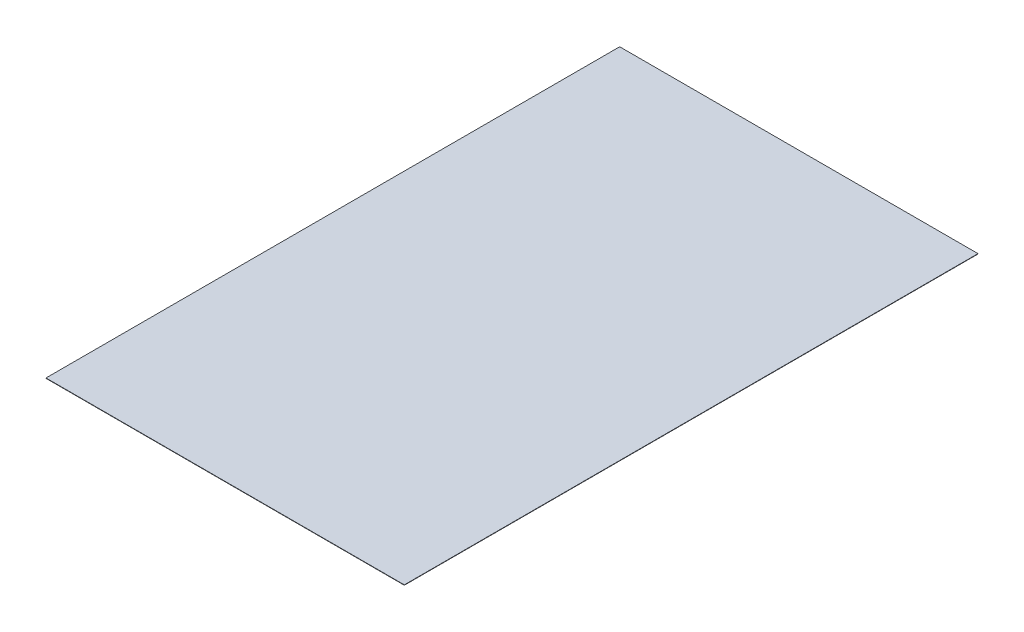
SolidWorks part; units mm, degrees
ref_plane "Front Plane" through (0, 0, 0) normal (0, 0, 1) x (1, 0, 0)
ref_plane "Top Plane" through (0, 0, 0) normal (0, 1, 0) x (1, 0, 0)
ref_plane "Right Plane" through (0, 0, 0) normal (1, 0, 0) x (0, 0, -1)
sketch "Sketch1" plane through (0, 0, 0) normal (0, 1, 0) x (1, 0, 0)
  line L1 (-500, -800.5) -> (500, -800.5)
  line L2 (-500, -800.5) -> (-500, 800.5)
  line L3 (-500, 800.5) -> (500, 800.5)
  line L4 (500, -800.5) -> (500, 800.5)
  line L5 (-500, -800.5) -> (500, 800.5) construction
  line L6 (-500, 800.5) -> (500, -800.5) construction
  point P0 (0, 0)
  dimension "D1" = 1000
  dimension "D2" = 1601
extrude "Boss-Extrude1" add sketch "Sketch1" along normal blind 1
